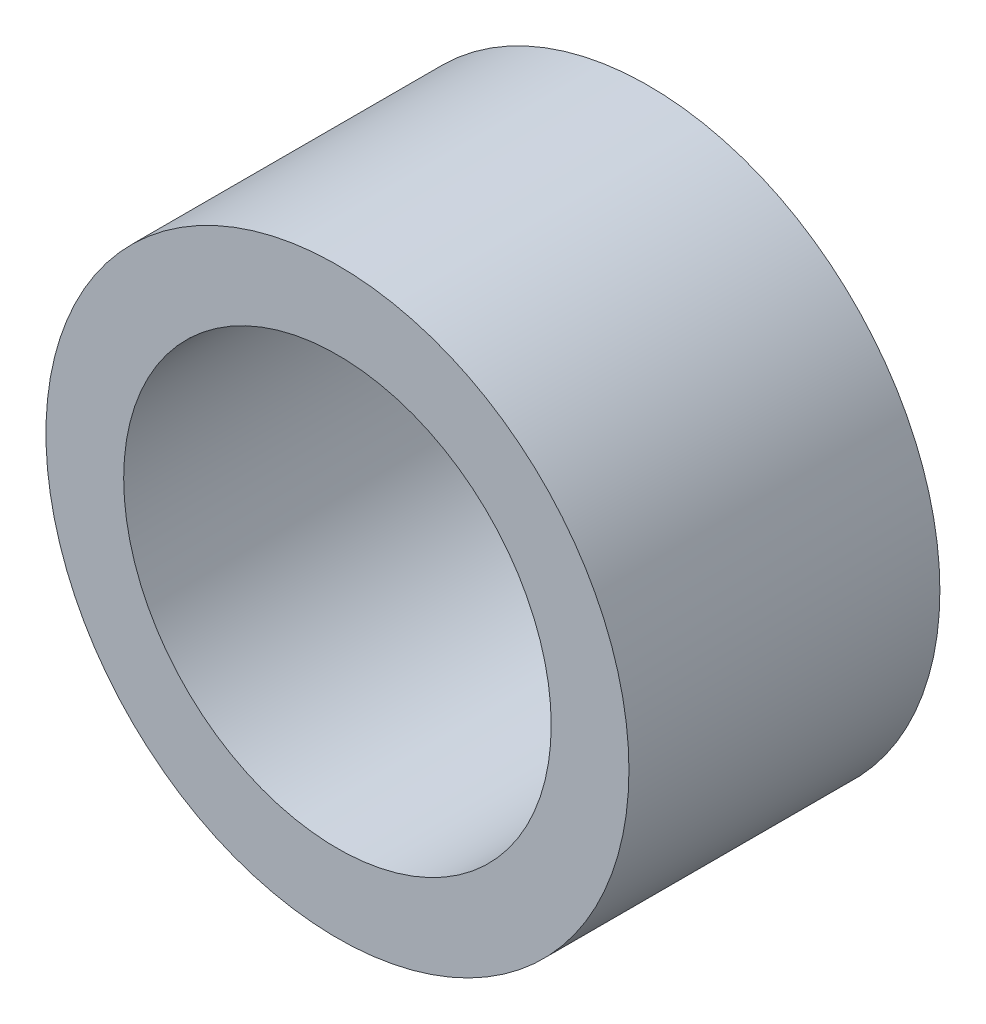
SolidWorks part; units mm, degrees
ref_plane "前视基准面" through (0, 0, 0) normal (0, 0, 1) x (1, 0, 0)
ref_plane "上视基准面" through (0, 0, 0) normal (0, 1, 0) x (1, 0, 0)
ref_plane "右视基准面" through (0, 0, 0) normal (1, 0, 0) x (0, 0, -1)
sketch "草图1" plane through (0, 0, 0) normal (0, 0, 1) x (1, 0, 0)
  circle A0 centre (0, 0) radius 5.5
  circle A1 centre (0, 0) radius 7.5
  dimension "D1" = 15
  dimension "D2" = 11
extrude "凸台-拉伸1" add sketch "草图1" along normal blind 8
